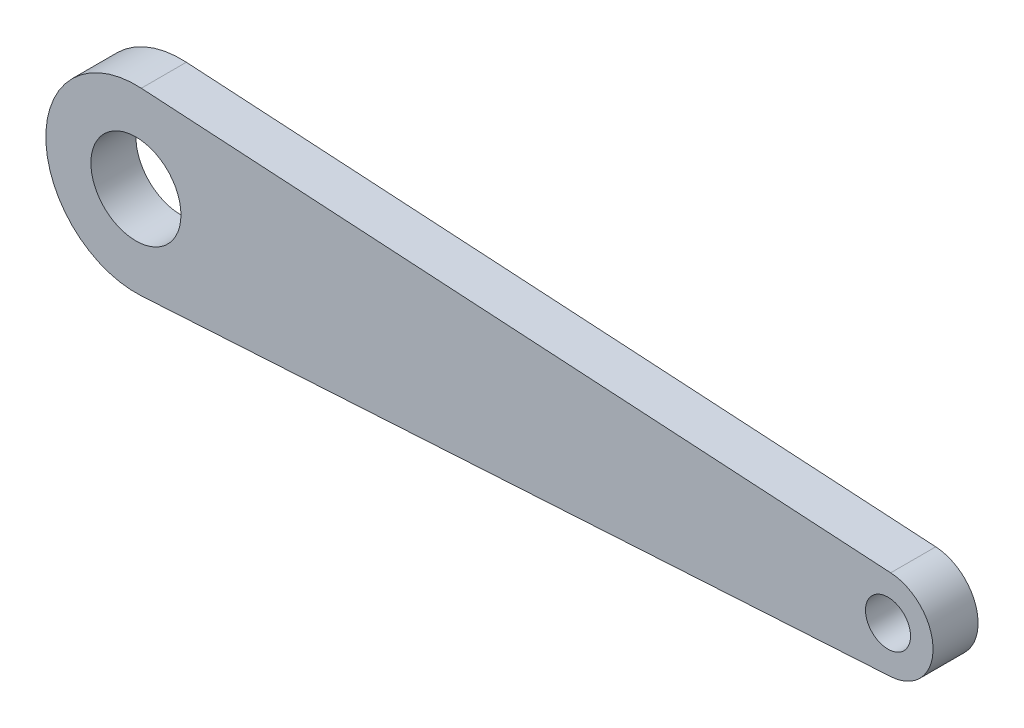
SolidWorks part; units mm, degrees
ref_plane "Front Plane" through (0, 0, 0) normal (0, 0, 1) x (1, 0, 0)
ref_plane "Top Plane" through (0, 0, 0) normal (0, 1, 0) x (1, 0, 0)
ref_plane "Right Plane" through (0, 0, 0) normal (1, 0, 0) x (0, 0, -1)
sketch "Sketch1" plane through (0, 0, 0) normal (0, 0, 1) x (1, 0, 0)
  line L0 (11.976, 199.6411) -> (1675.988, 99.8206)
  line L2 (11.976, -199.6411) -> (1675.988, -99.8206)
  arc A0 (11.976, 199.6411) -> (11.976, -199.6411) centre (0, 0) ccw
  arc A1 (1675.988, -99.8206) -> (1675.988, 99.8206) centre (1670, 0) ccw
  circle A2 centre (0, 0) radius 100
  circle A3 centre (1670, 0) radius 50
  dimension "D2" = 400
  dimension "D3" = 200
  dimension "D5" = 200
  dimension "D6" = 100
  dimension "D1" = 1670
  dimension "D4" = 0
extrude "Boss-Extrude1" add sketch "Sketch1" along normal blind 100
